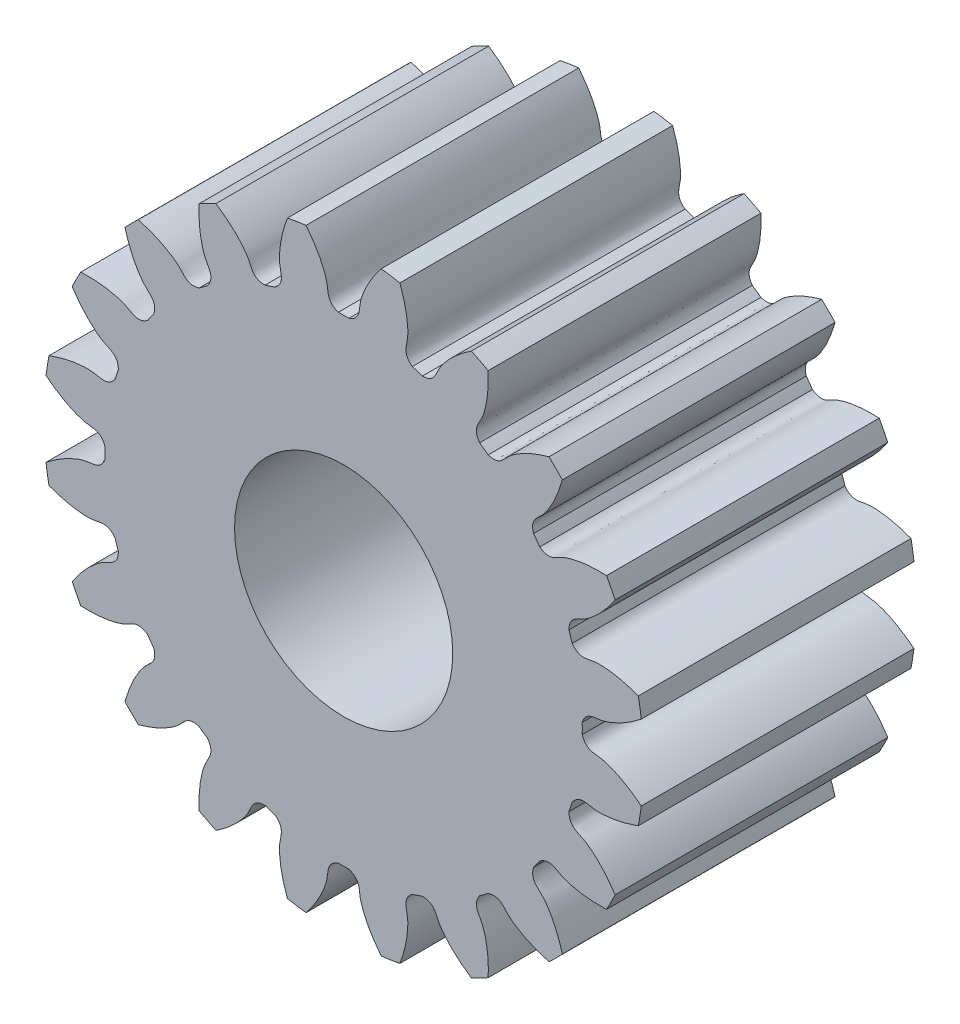
from build123d import *

# Parameters (mm, degrees)
SKETCH1_R           = 11
BOSS_EXTRUDE1_DEPTH = 10
CUT_EXTRUDE1_DEPTH  = 19.493242009
CIRPATTERN1_COUNT   = 20
SKETCH4_R           = 4
CUT_EXTRUDE2_DEPTH  = 19.390321144
CUT_EXTRUDE6_DEPTH  = 1.4


with BuildPart() as part:
    # Sketch1 → Boss-Extrude1 (new body)
    with BuildSketch(Plane.XY):
        Circle(SKETCH1_R)
    extrude(amount=BOSS_EXTRUDE1_DEPTH)

    # Sketch2 → Cut-Extrude1 (cut, through all)
    with BuildSketch(Plane.XY):
        with BuildLine():
            ThreePointArc((0.1933166, 8.747864236), (0, 8.75), (-0.1933166, 8.747864236))
            add(Edge.make_bspline(
                [(-0.1933166, 8.747864236), (-0.611189405, 8.893475512), (-0.557084099, 9.187113699), (-0.612897056, 9.470009403), (-0.618892186, 9.497556614), (-0.62631089, 9.528634615), (-0.635292097, 9.563196836), (-0.64597914, 9.601191497), (-0.658512055, 9.642562828), (-0.673029871, 9.687250733), (-0.68966975, 9.735190947), (-0.7085671, 9.786315045), (-0.729855399, 9.840550501), (-0.753666102, 9.897820731), (-0.780128531, 9.958045151), (-0.809369765, 10.021139231), (-0.841514533, 10.087014551), (-0.876685117, 10.155578861), (-0.915001238, 10.22673615), (-0.956579966, 10.300386704), (-1.001535609, 10.376427181), (-1.049979626, 10.454750678), (-1.102020521, 10.535246805), (-1.157763756, 10.617801764), (-1.217311651, 10.70229842), (-1.280763301, 10.78861639), (-1.34821448, 10.876632121), (-1.419757562, 10.966218973), (-1.495481426, 11.057247311), (-1.575471385, 11.149584594), (-1.659809097, 11.243095463), (-1.748572489, 11.337641835), (-1.841835684, 11.433083002), (-1.939668926, 11.529275727), (-2.042138506, 11.626074339), (-2.149306698, 11.723330842), (-2.261231689, 11.820895011), (-2.377967518, 11.918614499), (-2.499564012, 12.016334946), (-2.626066734, 12.113900082), (-2.757516899, 12.21115184), (-2.941473591, 12.341639868), (-3.083932413, 12.436332601), (-3.181157982, 12.49825186)],
                knots=[0, 0, 0, 0, 0.165916003, 0.170905922, 0.176663519, 0.183188797, 0.190481754, 0.198542391, 0.207370708, 0.216966704, 0.22733038, 0.238461736, 0.250360771, 0.263027487, 0.276461881, 0.290663956, 0.30563371, 0.321371144, 0.337876258, 0.355149051, 0.373189524, 0.391997677, 0.411573509, 0.431917021, 0.453028213, 0.474907084, 0.497553636, 0.520967867, 0.545149777, 0.570099367, 0.595816637, 0.622301587, 0.649554216, 0.677574526, 0.706362514, 0.735918183, 0.766241531, 0.797332559, 0.829191267, 0.861817654, 0.895211721, 0.929373468, 1, 1, 1, 1], degree=3))
            ThreePointArc((-3.181157982, 12.49825186), (0, 12.89674632), (3.181157982, 12.49825186))
            add(Edge.make_bspline(
                [(0.1933166, 8.747864236), (0.611189405, 8.893475512), (0.557084099, 9.187113699), (0.612897056, 9.470009403), (0.618892186, 9.497556614), (0.62631089, 9.528634615), (0.635292097, 9.563196836), (0.64597914, 9.601191497), (0.658512055, 9.642562828), (0.673029871, 9.687250733), (0.68966975, 9.735190947), (0.7085671, 9.786315045), (0.729855399, 9.840550501), (0.753666102, 9.897820731), (0.780128531, 9.958045151), (0.809369765, 10.021139231), (0.841514533, 10.087014551), (0.876685117, 10.155578861), (0.915001238, 10.22673615), (0.956579966, 10.300386704), (1.001535609, 10.376427181), (1.049979626, 10.454750678), (1.102020521, 10.535246805), (1.157763756, 10.617801764), (1.217311651, 10.70229842), (1.280763301, 10.78861639), (1.34821448, 10.876632121), (1.419757562, 10.966218973), (1.495481426, 11.057247311), (1.575471385, 11.149584594), (1.659809097, 11.243095463), (1.748572489, 11.337641835), (1.841835684, 11.433083002), (1.939668926, 11.529275727), (2.042138506, 11.626074339), (2.149306698, 11.723330842), (2.261231689, 11.820895011), (2.377967518, 11.918614499), (2.499564012, 12.016334946), (2.626066734, 12.113900082), (2.757516899, 12.21115184), (2.941473591, 12.341639868), (3.083932413, 12.436332601), (3.181157982, 12.49825186)],
                knots=[0, 0, 0, 0, 0.165916003, 0.170905922, 0.176663519, 0.183188797, 0.190481754, 0.198542391, 0.207370708, 0.216966704, 0.22733038, 0.238461736, 0.250360771, 0.263027487, 0.276461881, 0.290663956, 0.30563371, 0.321371144, 0.337876258, 0.355149051, 0.373189524, 0.391997677, 0.411573509, 0.431917021, 0.453028213, 0.474907084, 0.497553636, 0.520967867, 0.545149777, 0.570099367, 0.595816637, 0.622301587, 0.649554216, 0.677574526, 0.706362514, 0.735918183, 0.766241531, 0.797332559, 0.829191267, 0.861817654, 0.895211721, 0.929373468, 1, 1, 1, 1], degree=3))
        make_face()
    cut_extrude1 = extrude(amount=CUT_EXTRUDE1_DEPTH, mode=Mode.SUBTRACT)

    # CirPattern1: Cut-Extrude1 ×20 about axis
    cirpattern1_axis = Axis((0, 0, 10), (0, 0, -1))
    for i in range(1, CIRPATTERN1_COUNT):
        add(cut_extrude1.rotate(cirpattern1_axis, i * 360 / CIRPATTERN1_COUNT), mode=Mode.SUBTRACT)

    # Sketch4 → Cut-Extrude2 (cut, through all)
    with BuildSketch(Plane.XY.offset(10)):
        Circle(SKETCH4_R)
    extrude(amount=-CUT_EXTRUDE2_DEPTH, mode=Mode.SUBTRACT)

    # Sketch5 → Cut-Extrude6 (cut, symmetric)
    with BuildSketch(Plane(origin=(0, 4, 0), x_dir=(1, 0, 0), z_dir=(0, 1, 0))):
        with BuildLine():
            Line((1.5, -1.5), (1.5, -6.5))
            ThreePointArc((1.5, -6.5), (0, -8), (-1.5, -6.5))
            Line((-1.5, -6.5), (-1.5, -1.5))
            Line((-1.5, -1.5), (-1.5, 1.168792047))
            Line((-1.5, 1.168792047), (1.5, 1.168792047))
            Line((1.5, 1.168792047), (1.5, -1.5))
        make_face()
    extrude(amount=CUT_EXTRUDE6_DEPTH, both=True, mode=Mode.SUBTRACT)


solid = part.part
